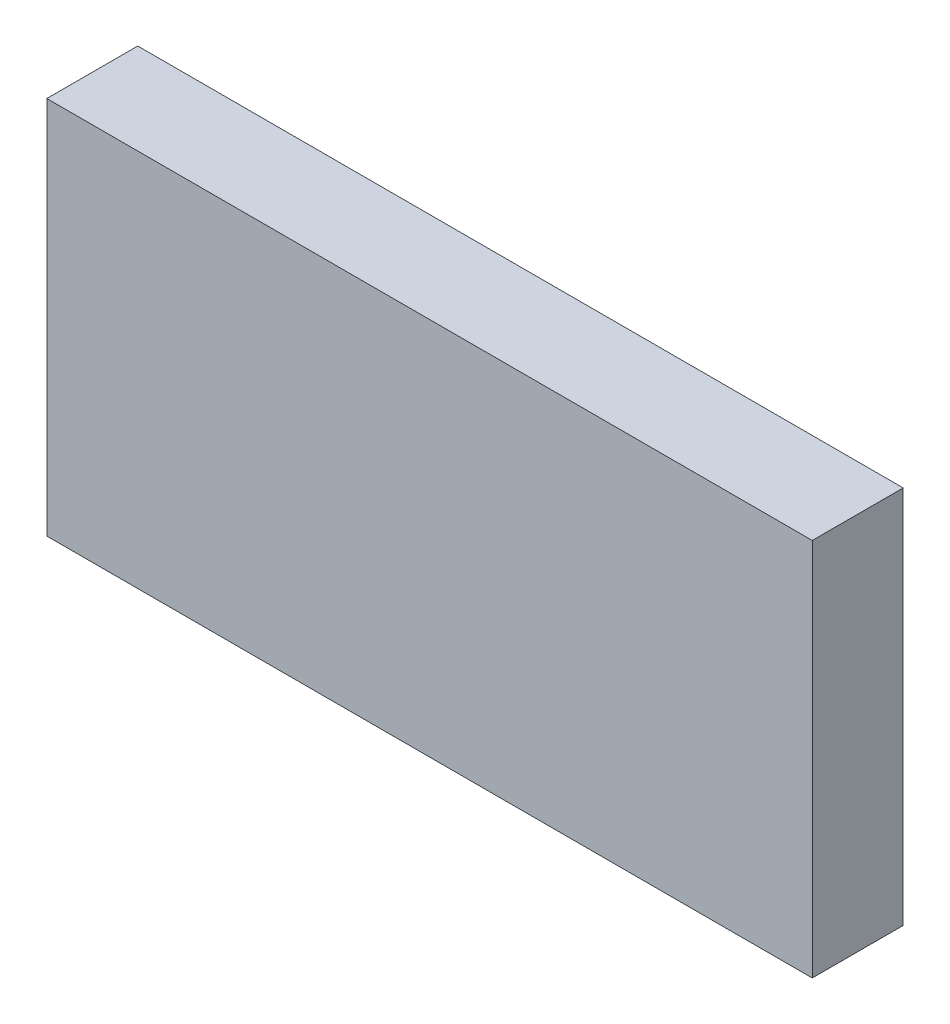
SolidWorks part; units mm, degrees
material "Q235B"
ref_plane "Front Plane" through (0, 0, 0) normal (0, 0, 1) x (1, 0, 0)
ref_plane "Top Plane" through (0, 0, 0) normal (0, 1, 0) x (1, 0, 0)
ref_plane "Right Plane" through (0, 0, 0) normal (1, 0, 0) x (0, 0, -1)
sketch "Sketch1" plane through (0, 0, 0) normal (0, 0, 1) x (1, 0, 0)
  line L1 (50.5, -25) -> (-50.5, -25)
  line L2 (50.5, -25) -> (50.5, 25)
  line L3 (50.5, 25) -> (-50.5, 25)
  line L4 (-50.5, -25) -> (-50.5, 25)
  line L5 (50.5, -25) -> (-50.5, 25) construction
  line L6 (50.5, 25) -> (-50.5, -25) construction
  point P0 (0, 0)
  dimension "D1" = 50
  dimension "D2" = 101
extrude "Boss-Extrude1" add sketch "Sketch1" along normal mid plane 12
